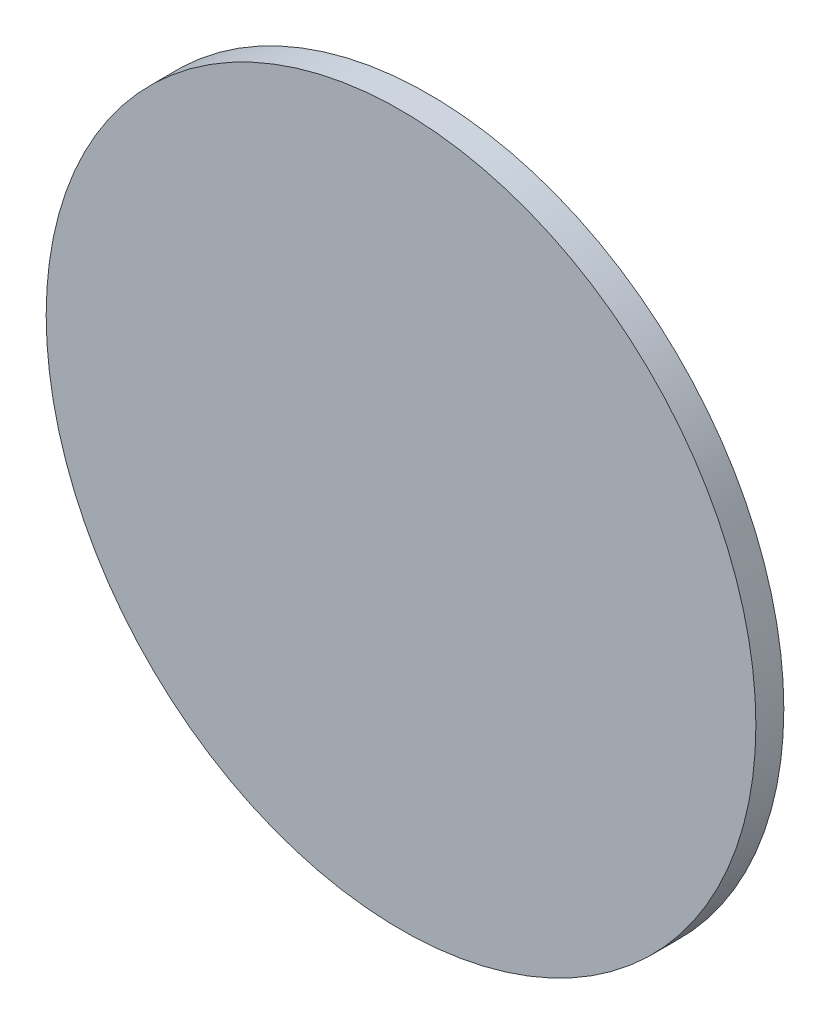
SolidWorks part; units mm, degrees
ref_plane "Front Plane" through (0, 0, 0) normal (0, 0, 1) x (1, 0, 0)
ref_plane "Top Plane" through (0, 0, 0) normal (0, 1, 0) x (1, 0, 0)
ref_plane "Right Plane" through (0, 0, 0) normal (1, 0, 0) x (0, 0, -1)
sketch "Sketch1" plane through (0, 0, 0) normal (0, 0, 1) x (1, 0, 0)
  circle A0 centre (28.2, -28.2) radius 12.7
  dimension "D1" = 25.4
extrude "Boss-Extrude1" add sketch "Sketch1" along normal blind 1
